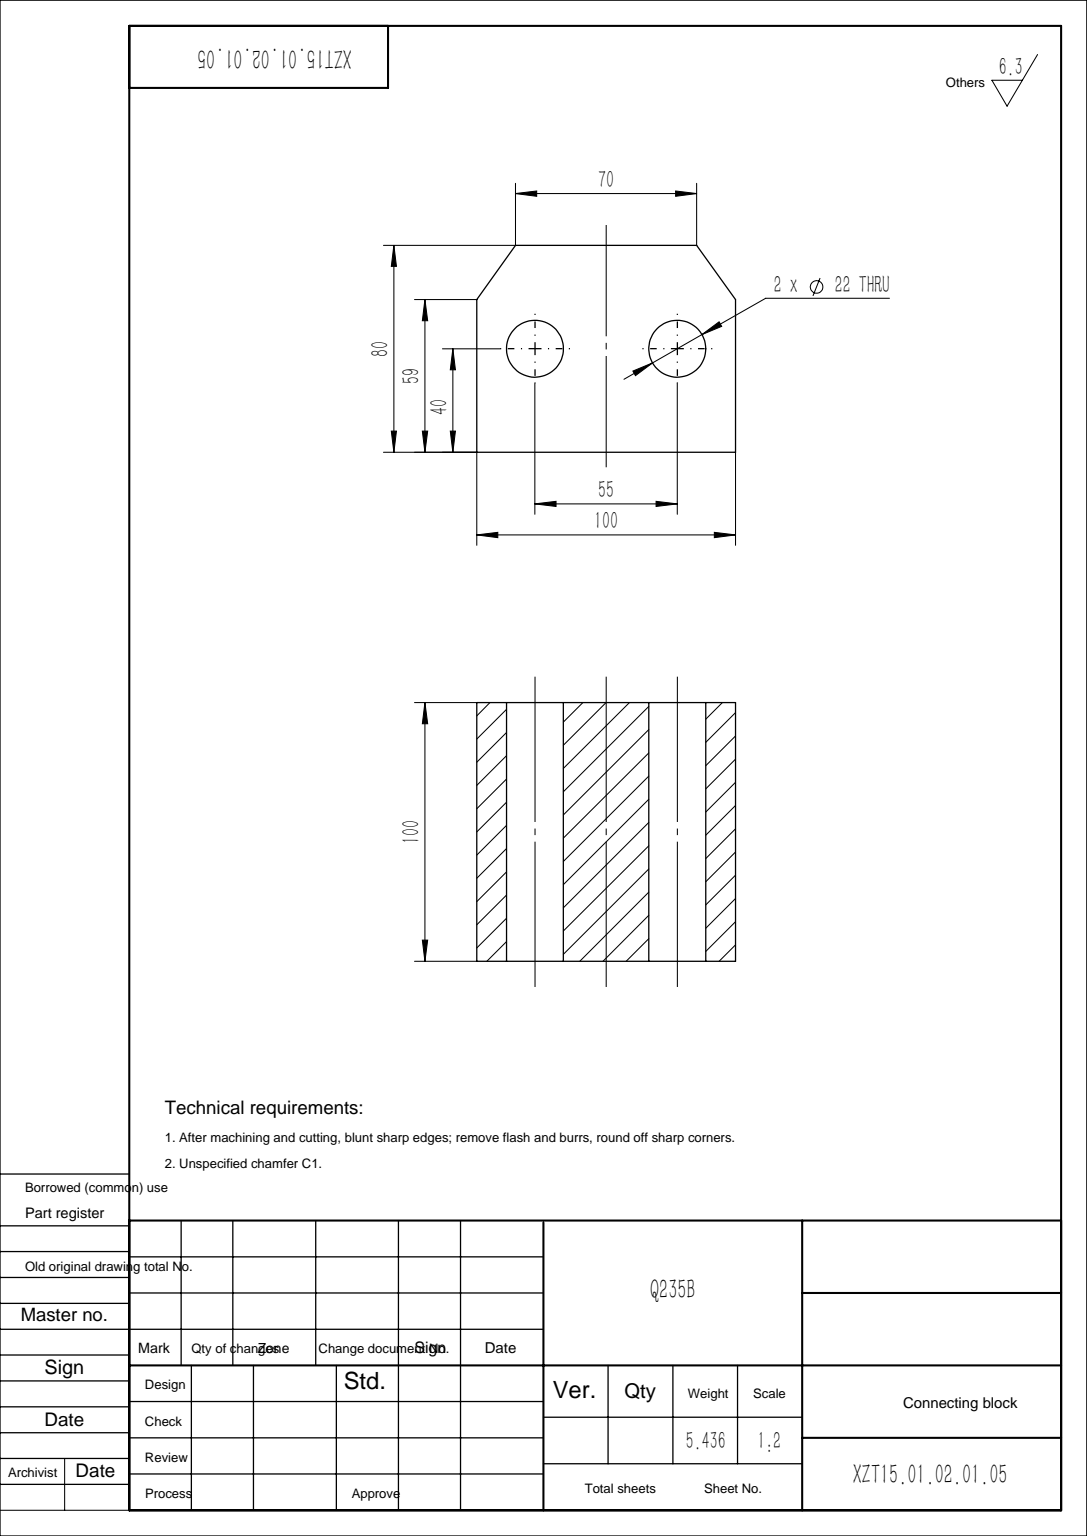
SolidWorks part; units mm, degrees
material "Q235B"
ref_plane "Front Plane" through (0, 0, 0) normal (0, 0, 1) x (1, 0, 0)
ref_plane "Top Plane" through (0, 0, 0) normal (0, 1, 0) x (1, 0, 0)
ref_plane "Right Plane" through (0, 0, 0) normal (1, 0, 0) x (0, 0, -1)
sketch "Sketch1" plane through (0, 0, 0) normal (0, 0, 1) x (1, 0, 0)
  line L1 (50, -40) -> (-50, -40)
  line L2 (50, -40) -> (50, 40)
  line L3 (50, 40) -> (-50, 40)
  line L4 (-50, -40) -> (-50, 40)
  line L5 (50, -40) -> (-50, 40) construction
  line L6 (50, 40) -> (-50, -40) construction
  point P0 (0, 0)
  dimension "D1" = 80
  dimension "D2" = 100
extrude "Boss-Extrude1" add sketch "Sketch1" along normal blind 100
chamfer "Chamfer1" distance 10 angle 45 2 edges at (-50, 40, 50) (50, 40, 50)
hole_wizard "Ø22 Diameter Hole1" positions "Sketch2" profile "Sketch3" hole size "Ø12.0" standard "GB" end condition up to next
sketch "Sketch2" plane through (0, 0, 100) normal (0, 0, 1) x (1, 0, 0)
  line L0 (0, 40) -> (0, -40) construction
  line L1 (40, 40) -> (-40, 40) construction
  line L2 (-50, -40) -> (50, -40) construction
  point P0 (-27.5, 0)
  point P10 (27.5, 0)
  dimension "D1" = 55
  dimension "D2" = 40
sketch "Sketch3" plane through (-27.5, 0, 100) normal (1, 0, 0) x (0, -1, 0)
  line L0 (0, 0) -> (0, 100)
  line L1 (0, 100) -> (11, 100)
  line L2 (11, 100) -> (11, 0)
  line L5 (11, 0) -> (0, 0)
  line L11 (0, -6.35) -> (0, 107.95) construction
  dimension "通孔孔直径" = 22
  dimension "通孔孔深度" = 100
sketch "Sketch4" plane through (0, 0, 100) normal (0, 0, 1) x (1, 0, 0)
  line L0 (-35, 40) -> (-50, 19)
  line L1 (40, 40) -> (-40, 40) construction
  line L2 (-50, 30) -> (-50, -40) construction
  line L3 (-50, 19) -> (-50, 40)
  line L4 (-50, 40) -> (-35, 40)
  line L5 (0, 40) -> (0, 0) construction
  line L6 (50, 40) -> (35, 40)
  line L7 (50, 19) -> (50, 40)
  line L8 (35, 40) -> (50, 19)
  line L9 (-50, -40) -> (50, -40) construction
  dimension "D1" = 70
  dimension "D2" = 59
extrude "Cut-Extrude1" cut sketch "Sketch4" against normal through all both and the other way through all
